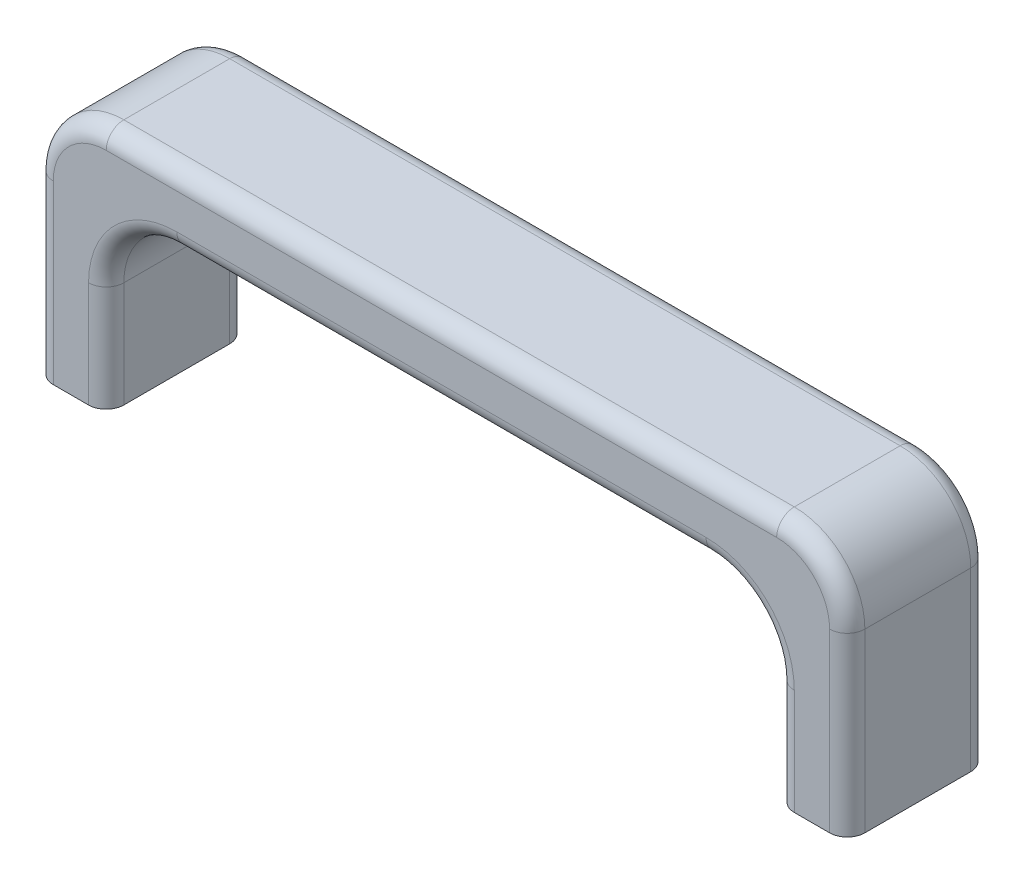
SolidWorks part; units mm, degrees
ref_plane "Front Plane" through (0, 0, 0) normal (0, 0, 1) x (1, 0, 0)
ref_plane "Top Plane" through (0, 0, 0) normal (0, 1, 0) x (1, 0, 0)
ref_plane "Right Plane" through (0, 0, 0) normal (1, 0, 0) x (0, 0, -1)
other "Configuration Table"
sketch "Sketch1" plane through (0, 0, 0) normal (0, 0, 1) x (1, 0, 0)
  line L0 (-41, 226) -> (-41, 296)
  line L1 (-41, 296) -> (189, 296)
  line L2 (189, 296) -> (189, 226)
  line L3 (-21, 226) -> (-21, 276)
  line L4 (-21, 276) -> (169, 276)
  line L5 (169, 276) -> (169, 226)
  line L6 (-21, 226) -> (-41, 226)
  line L7 (189, 226) -> (169, 226)
  dimension "D1" = 70
  dimension "D2" = 20
extrude "Boss-Extrude1" add sketch "Sketch1" along normal mid plane 40 contours L3 L4 L5 L7 L2 L1 L0 L6
fillet "Fillet1" radius 20 4 edges at (189, 296, 0) (169, 276, 0) (-21, 276, 0) (-41, 296, 0)
fillet "Fillet2" radius 5 20 edges at (-41, 251, -20) (-35.1421, 290.1421, -20) (189, 251, -20) (183.1421, 290.1421, -20) (-41, 251, 20) (-35.1421, 290.1421, 20) (189, 251, 20) (183.1421, 290.1421, 20) (74, 296, -20) (74, 296, 20) (169, 241, -20) (163.1421, 270.1421, -20) (74, 276, -20) (-15.1421, 270.1421, -20) (169, 241, 20) (163.1421, 270.1421, 20) (74, 276, 20) (-15.1421, 270.1421, 20) (-21, 241, -20) (-21, 241, 20)
hole_wizard "M10 Tapped Hole1" positions "3DSketch1" profile "Sketch2" tap size "M10" standard "GB"
sketch3d "3DSketch1"
  line L0 (-26, 226, 20) -> (-36, 226, 20) construction
  line L1 (-41, 226, 15) -> (-41, 226, -15) construction
  line L3 (184, 226, 20) -> (174, 226, 20) construction
  point P0 (-31, 226, 0)
  point P2 (179, 226, 0)
  point P8 (-31, 226, 20)
  point P11 (-41, 226, 0)
  point P16 (179, 226, 20)
sketch "Sketch2" plane through (-31, 226, 0) normal (1, 0, 0) x (0, 0, -1)
  line L0 (0, 0) -> (0, 27.5537)
  line L1 (0, 27.5537) -> (4.25, 25)
  line L2 (4.25, 25) -> (4.25, 0.775)
  line L3 (4.25, 0.775) -> (5.025, 0)
  line L5 (5.025, 0) -> (0, 0)
  line L6 (-4.25, 0.775) -> (-5.025, 0) construction
  line L10 (0, 27.5537) -> (-4.25, 25) construction
  line L11 (0, -6.35) -> (0, 107.95) construction
  dimension "螺纹孔钻头直径" = 8.5
  dimension "螺纹孔钻头深度" = 25
  dimension "近端锥形沉头孔直径" = 10.05
  dimension "近端锥形沉头孔角度" = 90
  dimension "导头角度" = 118
cosmetic thread "Cosmetic Thread1" parameters "D1"=20, "D2"=10
cosmetic thread "Cosmetic Thread2" parameters "D1"=20, "D2"=10
